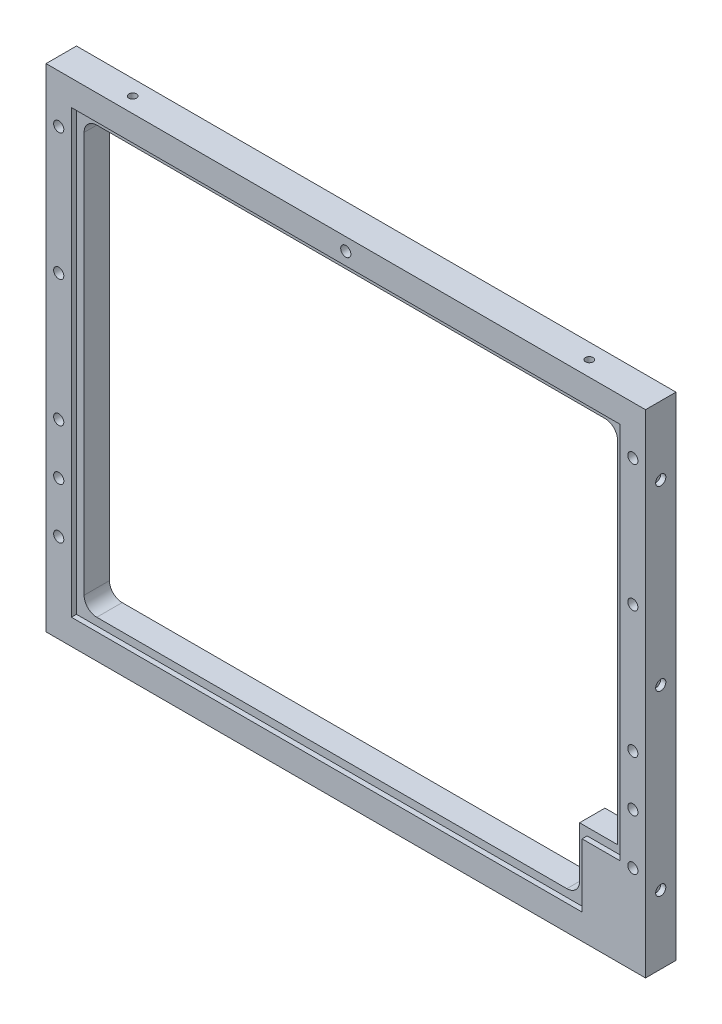
SolidWorks part; units mm, degrees
ref_plane "Front Plane" through (0, 0, 0) normal (0, 0, 1) x (1, 0, 0)
ref_plane "Top Plane" through (0, 0, 0) normal (0, 1, 0) x (1, 0, 0)
ref_plane "Right Plane" through (0, 0, 0) normal (1, 0, 0) x (0, 0, -1)
sketch "Sketch1" plane through (0, 0, 0) normal (0, 0, 1) x (1, 0, 0)
  line L1 (-118.15, 97) -> (118.15, 97)
  line L2 (-118.15, 97) -> (-118.15, -97)
  line L3 (-118.15, -97) -> (118.15, -97)
  line L4 (118.15, 97) -> (118.15, -97)
  line L5 (-118.15, 97) -> (118.15, -97) construction
  line L6 (-118.15, -97) -> (118.15, 97) construction
  point P0 (0, 0)
  dimension "D1" = 236.3
  dimension "D2" = 194
extrude "Boss-Extrude1" add sketch "Sketch1" along normal mid plane 12
sketch "Sketch2" plane through (0, 0, 6) normal (0, 0, 1) x (1, 0, 0)
  line L0 (-118.15, -97) -> (118.15, -97) construction
  line L1 (-108.15, 87) -> (108.15, 87)
  line L2 (-108.15, 87) -> (-108.15, -87)
  line L3 (-108.15, -87) -> (108.15, -87)
  line L4 (108.15, 87) -> (108.15, -87)
  line L5 (-108.15, 87) -> (108.15, -87) construction
  line L6 (-108.15, -87) -> (108.15, 87) construction
  line L7 (118.15, -97) -> (118.15, 97) construction
  line L8 (108.15, -62) -> (93.15, -62)
  line L9 (93.15, -62) -> (93.15, -87)
  point P0 (0, 0)
  dimension "D1" = 10
  dimension "D2" = 10
  dimension "D3" = 15
  dimension "D4" = 25
extrude "Cut-Extrude1" cut sketch "Sketch2" against normal blind 2 contours L9 L8 L4 L1 L2 L3
sketch "Sketch3" plane through (0, 0, 4) normal (0, 0, 1) x (1, 0, 0)
  line L12 (90.15, -84) -> (90.15, -59)
  line L13 (90.15, -59) -> (105.15, -59)
  line L14 (105.15, -59) -> (105.15, 84)
  line L15 (105.15, 84) -> (-105.15, 84)
  line L16 (-105.15, 84) -> (-105.15, -84)
  line L17 (-105.15, -84) -> (90.15, -84)
  line L18 (90.15, -84) -> (90.15, -59)
  line L19 (90.15, -59) -> (105.15, -59)
  line L20 (105.15, -59) -> (105.15, 84)
  line L21 (105.15, 84) -> (-105.15, 84)
  line L22 (-105.15, 84) -> (-105.15, -84)
  line L23 (-105.15, -84) -> (90.15, -84)
  dimension "D1" = 3
extrude "Cut-Extrude2" cut sketch "Sketch3" against normal through all
fillet "Fillet1" radius 5 4 edges at (90.15, -84, -1) (105.15, 84, -1) (-105.15, 84, -1) (-105.15, -84, -1)
sketch "Sketch4" plane through (-118.15, 0, 0) normal (-1, 0, 0) x (0, 0, 1)
  line L0 (0, 109.3519) -> (0, -123.4422) construction
  line L1 (-19.2448, 0) -> (21.1341, 0) construction
  circle A0 centre (0, 0) radius 2
  circle A1 centre (0, 70) radius 2
  circle A2 centre (0, -70) radius 2
  dimension "D1" = 4
  dimension "D2" = 4
  dimension "D3" = 70
extrude "Cut-Extrude3" cut sketch "Sketch4" against normal blind 2
mirror "Mirror1" about plane through (0, 0, 0) normal (1, 0, 0) of "Cut-Extrude3"
sketch "Sketch5" plane through (0, 97, 0) normal (0, 1, 0) x (1, 0, 0)
  line L0 (-130.753, 0) -> (128.1602, 0) construction
  line L1 (0, 24.0844) -> (0, -28.8835) construction
  circle A0 centre (-90, 0) radius 1.5
  circle A1 centre (90, 0) radius 1.5
  dimension "D1" = 3
  dimension "D2" = 90
extrude "Cut-Extrude4" cut sketch "Sketch5" against normal blind 4
mirror "Mirror2" about plane through (0, 0, 0) normal (0, 1, 0) of "Cut-Extrude4"
sketch "Sketch7" plane through (0, 0, 6) normal (0, 0, 1) x (1, 0, 0)
  line L0 (-118.15, 97) -> (-118.15, -97) construction
  line L1 (-118.15, -97) -> (118.15, -97) construction
  circle A0 centre (-113.15, 78) radius 2
  circle A1 centre (-113.15, 28) radius 2
  circle A2 centre (-113.15, -22) radius 2
  circle A3 centre (-113.15, -42) radius 2
  circle A4 centre (-113.15, -62) radius 2
  dimension "D1" = 4
  dimension "D2" = 4
  dimension "D3" = 4
  dimension "D4" = 4
  dimension "D5" = 4
  dimension "D6" = 5
  dimension "D7" = 35
  dimension "D8" = 20
  dimension "D9" = 20
  dimension "D10" = 50
  dimension "D11" = 50
extrude "Cut-Extrude6" cut sketch "Sketch7" against normal blind 4
mirror "Mirror3" about plane through (0, 0, 0) normal (1, 0, 0) of "Cut-Extrude6"
sketch "Sketch8" plane through (0, 0, 6) normal (0, 0, 1) x (1, 0, 0)
  line L0 (118.15, 97) -> (-118.15, 97) construction
  circle A0 centre (0, 92) radius 2
  dimension "D1" = 4
  dimension "D2" = 5
extrude "Cut-Extrude7" cut sketch "Sketch8" against normal blind 4
